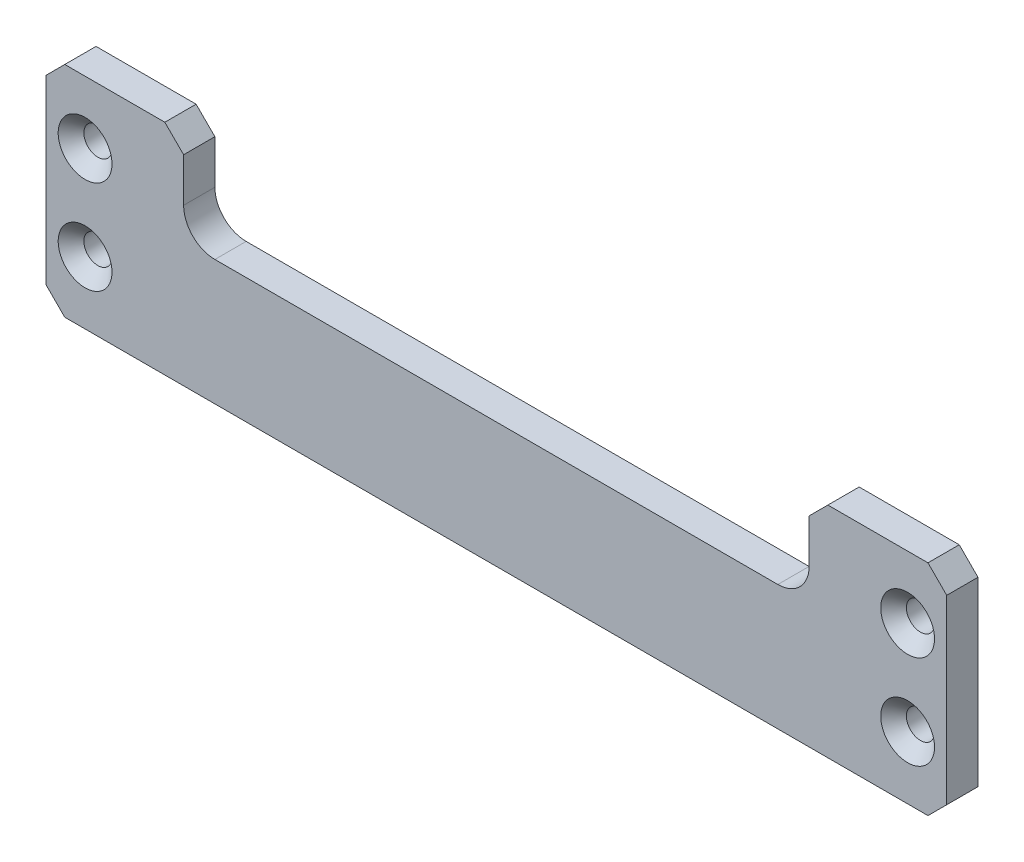
from build123d import *

# Parameters (mm, degrees)
SKETCH_1_W                = 144
SKETCH_1_H                = 35
EXTRUDE_1_DEPTH           = 5
HOLE_WIZARD_1_D           = 4.5
HOLE_WIZARD_1_CSINK_D     = 8.6
HOLE_WIZARD_1_CSINK_ANGLE = 90
SKETCH_4_W                = 100
SKETCH_4_H                = 15
CUT_EXTRUDE_1_DEPTH       = 75.264729179
CHAMFER_1_SIZE            = 3
FILLET_1_R                = 5


with BuildPart() as part:
    # 草图1 → 凸台-拉伸1 (new body)
    with BuildSketch(Plane.XY):
        Rectangle(SKETCH_1_W, SKETCH_1_H)
    extrude(amount=EXTRUDE_1_DEPTH)

    # 打孔尺寸根据十字槽沉头木螺钉的类型1 (through all)
    with Locations(Plane.XY.offset(5)):
        with Locations((-65.75, 7.5), (-65.75, -7.5), (65.75, 7.5), (65.75, -7.5)):
            CounterSinkHole(HOLE_WIZARD_1_D / 2, HOLE_WIZARD_1_CSINK_D / 2, counter_sink_angle=HOLE_WIZARD_1_CSINK_ANGLE)

    # 草图4 → 切除-拉伸1 (cut, through all)
    with BuildSketch(Plane.XY.offset(5)):
        with Locations((0, 10)):
            Rectangle(SKETCH_4_W, SKETCH_4_H)
    extrude(amount=-CUT_EXTRUDE_1_DEPTH, mode=Mode.SUBTRACT)

    # 倒角1
    chamfer_1_edges = [part.edges().sort_by_distance(p)[0] for p in [
        (-50, 17.5, 2.5),
        (50, 17.5, 2.5),
        (72, -17.5, 2.5),
        (-72, -17.5, 2.5),
        (-72, 17.5, 2.5),
        (72, 17.5, 2.5),
    ]]
    chamfer(chamfer_1_edges, length=CHAMFER_1_SIZE)

    # 圆角1
    fillet_1_edges = [part.edges().sort_by_distance(p)[0] for p in [
        (-50, 2.5, 2.5),
        (50, 2.5, 2.5),
    ]]
    fillet(fillet_1_edges, radius=FILLET_1_R)


solid = part.part
